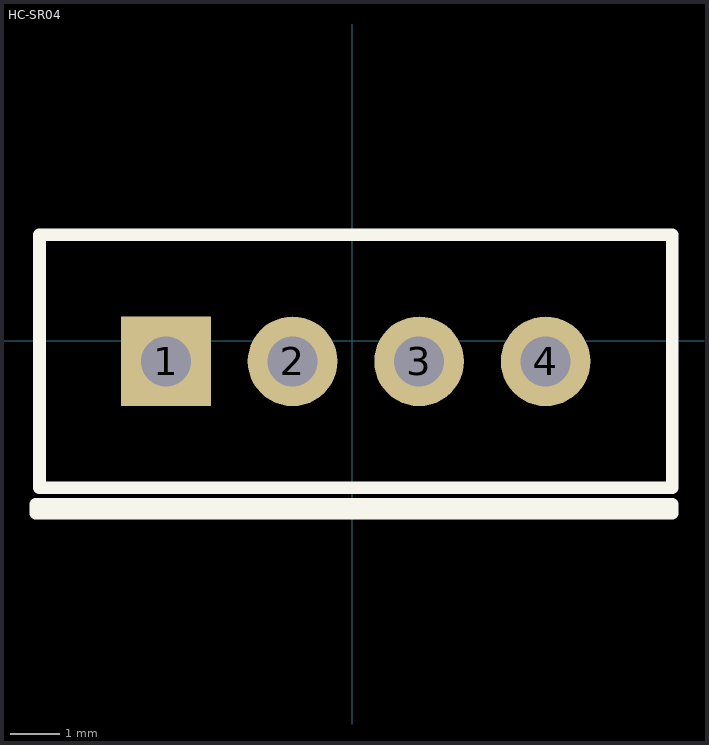
[diagram p0: the footprint, top view; thin cyan lines are the x and y axes]
# Altium footprint library MISC84237-11.PcbLib: 1 footprints
Each footprint in its own frame and in the unit in brackets; x right, y up, seen from the top. Pads: shape width x height; smd on the part's side, far side on the other; paste and mask are expansions set on the pad; w line width, h text height; cw(c..) or ccw(c..) is an arc to the next point about the centre after c.

## HC-SR04 [mm]
pads (4):
  rect 1.8x1.8 hole 1 paste+0 mask+0.102: 1(-3.742,-0.411)
  round 1.8 hole 1 paste+0 mask+0.102: 2(-1.202,-0.411) 3(1.338,-0.411) 4(3.878,-0.411)
Top Overlay:
  lines w0.254: -6.356,-3.459 -6.356,-3.286 6.418,-3.286 6.418,-3.459 -6.356,-3.459 ; -6.282,-2.951 -6.282,2.129 6.418,2.129 6.418,-2.951 -6.282,-2.951